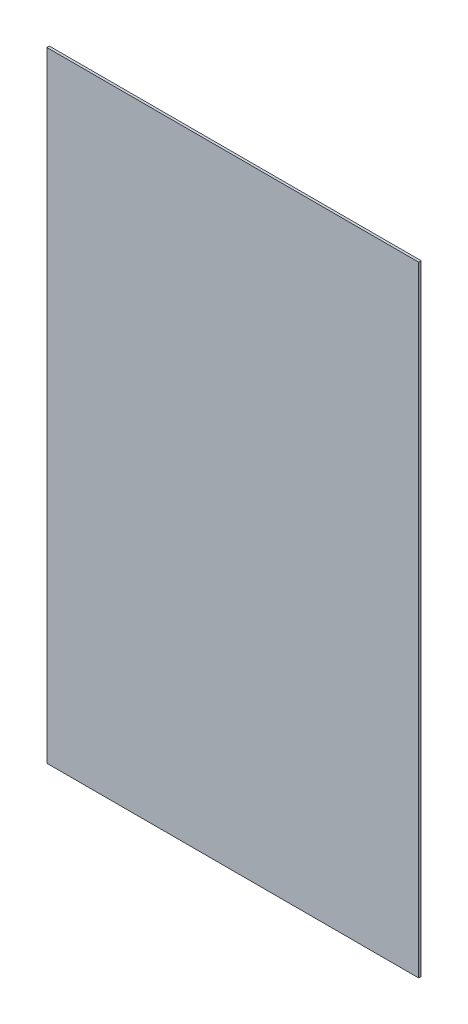
SolidWorks part; units mm, degrees
ref_plane "前视基准面" through (0, 0, 0) normal (0, 0, 1) x (1, 0, 0)
ref_plane "上视基准面" through (0, 0, 0) normal (0, 1, 0) x (1, 0, 0)
ref_plane "右视基准面" through (0, 0, 0) normal (1, 0, 0) x (0, 0, -1)
sketch "草图1" plane through (0, 0, 0) normal (0, 0, 1) x (1, 0, 0)
  line L1 (-15, -25) -> (15, -25)
  line L2 (-15, -25) -> (-15, 25)
  line L3 (-15, 25) -> (15, 25)
  line L4 (15, -25) -> (15, 25)
  line L5 (-15, -25) -> (15, 25) construction
  line L6 (-15, 25) -> (15, -25) construction
  text T0 "AOV" font "仿宋_GB" height 3.5
  point P0 (0, 0)
  dimension "D1" = 50
  dimension "D2" = 30
extrude "凸台-拉伸1" add sketch "草图1" along normal blind 0.2 contours L1 L4 L3 L2
